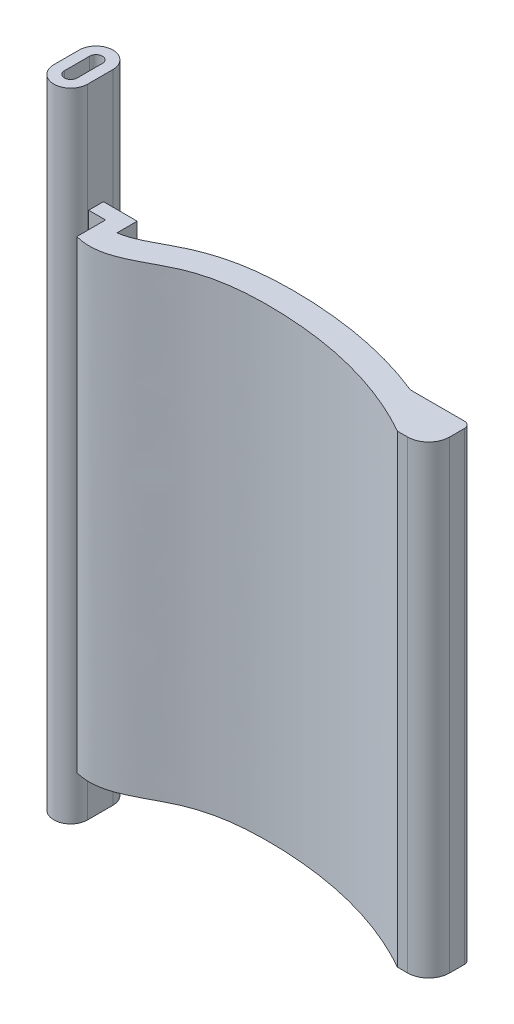
from build123d import *

# Parameters (mm, degrees)
EXTRUDE_THIN1_DEPTH      = 2
EXTRUDE_THIN1_DEPTH_BACK = 300
BOSS_EXTRUDE1_START      = -50
BOSS_EXTRUDE1_DEPTH      = 220


with BuildPart() as part:
    # Sketch1 → Extrude-Thin1 (new, two sides: drawn at the far end of the back side and taken through both)
    with BuildSketch(Plane(origin=(0, 0, 0), x_dir=(1, 0, 0), z_dir=(0, 1, 0)).offset(-EXTRUDE_THIN1_DEPTH_BACK)):
        with BuildLine():
            Line((-8, -0.503225806), (-8, 11.496774194))
            ThreePointArc((-8, 11.496774194), (0, 19.496774194), (8, 11.496774194))
            Line((8, 11.496774194), (8, -0.503225806))
            ThreePointArc((8, -0.503225806), (0, -8.503225806), (-8, -0.503225806))
        make_face()
        with BuildLine():
            Line((-3, -0.503225806), (-3, 11.496774194))
            ThreePointArc((-3, 11.496774194), (0, 14.496774194), (3, 11.496774194))
            Line((3, 11.496774194), (3, -0.503225806))
            ThreePointArc((3, -0.503225806), (0, -3.503225806), (-3, -0.503225806))
        make_face(mode=Mode.SUBTRACT)
    extrude(amount=EXTRUDE_THIN1_DEPTH + EXTRUDE_THIN1_DEPTH_BACK)

    # Sketch3 → Boss-Extrude1 (add)
    with BuildSketch(Plane(origin=(0, 0, 0), x_dir=(1, 0, 0), z_dir=(0, 1, 0)).offset(BOSS_EXTRUDE1_START)):
        with BuildLine():
            Line((8, 0), (16, 0))
            Line((16, 0), (16, -13.621259212))
            add(Edge.make_bspline(
                [(16, -13.621259212), (30.499922351, -17.644570766), (51.936419213, 1.310573607), (107.30973254, 6.157280303), (147.096775614, -3.484939683), (171.849245201, -17.511543594)],
                knots=[0, 0, 0, 0, 0.250267885, 0.483180841, 1, 1, 1, 1], degree=3))
            Line((171.849245201, -17.511543594), (176.613232431, -17.511543594))
            ThreePointArc((176.613232431, -17.511543594), (183.684300243, -14.582611406), (186.613232431, -7.511543594))
            Line((186.613232431, -7.511543594), (186.613232431, -0.511543594))
            ThreePointArc((186.613232431, -0.511543594), (185.734552774, 1.60977675), (183.613232431, 2.488456406))
            Line((183.613232431, 2.488456406), (158, 2.488456406))
            add(Edge.make_bspline(
                [(24, -2.514580028), (24.113004411, -2.504983511), (24.349957742, -2.482060724), (25.509506663, -2.341745989), (27.600697432, -1.88324406), (31.010172468, -0.626291734), (34.87998125, 1.213798693), (39.186324623, 3.500572248), (43.160103091, 5.617485681), (46.601418923, 7.314594934), (49.348560323, 8.562999499), (52.193103542, 9.711388614), (55.982687982, 11.062684309), (60.757798847, 12.456180642), (66.494574497, 13.702828567), (74.121472863, 14.874668238), (81.665278055, 15.420557925), (89.055802359, 15.540070459), (96.311727988, 15.442620679), (105.361571511, 14.955938635), (119.728798439, 13.363447087), (136.566579979, 9.992440329), (150.375206962, 5.520091676), (157.156359053, 2.830882837), (158, 2.488456406)],
                knots=[0.05434909, 0.05434909, 0.05434909, 0.05434909, 0.05825534, 0.0625, 0.09375, 0.125, 0.15625, 0.1875, 0.21875, 0.234375, 0.25, 0.265625, 0.28125, 0.3125, 0.34375, 0.375, 0.4375, 0.46875, 0.5, 0.5625, 0.625, 0.75, 0.859647043, 0.875272043, 0.875272043, 0.875272043, 0.875272043], degree=3))
            Line((24, -2.514580028), (24, 7))
            Line((24, 7), (8, 7))
            Line((8, 7), (8, 0))
        make_face()
    extrude(amount=-BOSS_EXTRUDE1_DEPTH)


solid = part.part
